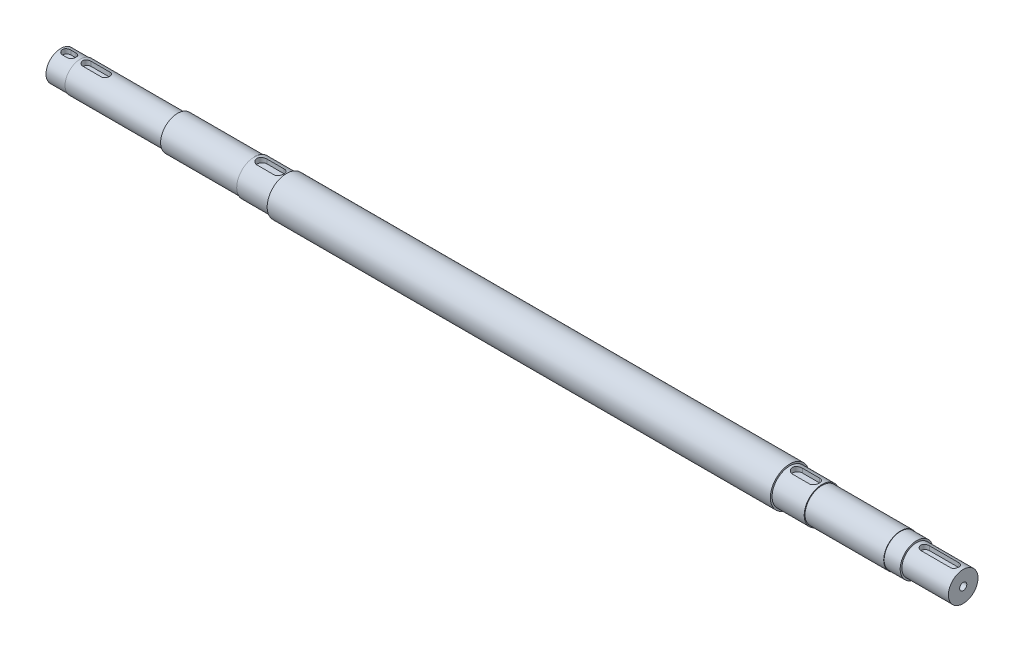
SolidWorks part; units mm, degrees
material "45"
ref_plane "前视基准面" through (0, 0, 0) normal (0, 0, 1) x (1, 0, 0)
ref_plane "上视基准面" through (0, 0, 0) normal (0, 1, 0) x (1, 0, 0)
ref_plane "右视基准面" through (0, 0, 0) normal (1, 0, 0) x (0, 0, -1)
sketch "草图1" plane through (0, 0, 0) normal (1, 0, 0) x (0, 0, -1)
  circle A0 centre (0, 0) radius 23
extrude "凸台-拉伸1" add sketch "草图1" along normal blind 595
sketch "草图2" plane through (0, 0, 0) normal (-1, 0, 0) x (0, 0, 1)
  circle A0 centre (0, 0) radius 21
extrude "凸台-拉伸2" add sketch "草图2" along normal blind 38
sketch "草图3" plane through (-38, 0, 0) normal (-1, 0, 0) x (0, 0, 1)
  circle A0 centre (0, 0) radius 20
extrude "凸台-拉伸3" add sketch "草图3" along normal blind 91
sketch "草图4" plane through (-129, 0, 0) normal (-1, 0, 0) x (0, 0, 1)
  circle A0 centre (0, 0) radius 18
extrude "凸台-拉伸4" add sketch "草图4" along normal blind 115
sketch "草图5" plane through (-244, 0, 0) normal (-1, 0, 0) x (0, 0, 1)
  circle A0 centre (0, 0) radius 17.5
extrude "凸台-拉伸5" add sketch "草图5" along normal blind 23
ref_plane "基准面1" through (0, 21, 0) normal (0, 1, 0) x (1, 0, 0)
sketch "草图6" plane through (0, 21, 0) normal (0, 1, 0) x (1, 0, 0)
  line L0 (-9, 0) -> (-29, 0) construction
  line L1 (-9, -6) -> (-29, -6)
  line L2 (-9, 6) -> (-29, 6)
  line L3 (0, 21) -> (0, -21) construction
  line L4 (604, 0) -> (624, 0) construction
  line L5 (595, -23) -> (595, 23) construction
  line L6 (604, 6) -> (624, 6)
  line L7 (604, -6) -> (624, -6)
  arc A0 (-9, -6) -> (-9, 6) centre (-9, 0) ccw
  arc A1 (-29, 6) -> (-29, -6) centre (-29, 0) ccw
  arc A2 (604, 6) -> (604, -6) centre (604, 0) ccw
  arc A3 (624, -6) -> (624, 6) centre (624, 0) ccw
  point P3 (-19, 0)
  point P14 (614, 0)
  dimension "D1" = 9
  dimension "D2" = 6
  dimension "D4" = 20
  dimension "D5" = 6
  dimension "D3" = 20
  dimension "D6" = 9
sketch "草图7" plane through (595, 0, 0) normal (1, 0, 0) x (0, 0, -1)
  circle A0 centre (0, 0) radius 21
extrude "凸台-拉伸6" add sketch "草图7" along normal blind 38
extrude "切除-拉伸2" cut sketch "草图6" against normal blind 5.88
ref_plane "基准面2" through (0, 18, 0) normal (0, 1, 0) x (1, 0, 0)
sketch "草图9" plane through (0, 18, 0) normal (0, 1, 0) x (1, 0, 0)
  line L0 (-236, 0) -> (-214, 0) construction
  line L1 (-244, 18) -> (-244, -18) construction
  line L2 (-236, 5) -> (-214, 5)
  line L3 (-236, -5) -> (-214, -5)
  arc A0 (-236, 5) -> (-236, -5) centre (-236, 0) ccw
  arc A1 (-214, -5) -> (-214, 5) centre (-214, 0) ccw
  point P5 (-225, 0)
  dimension "D1" = 22
  dimension "D2" = 5
  dimension "D3" = 8
extrude "切除-拉伸3" cut sketch "草图9" against normal blind 6.03
sketch "草图10" plane through (633, 0, 0) normal (1, 0, 0) x (0, 0, -1)
  circle A0 centre (0, 0) radius 20
extrude "凸台-拉伸7" add sketch "草图10" along normal blind 93
sketch "草图11" plane through (726, 0, 0) normal (1, 0, 0) x (0, 0, -1)
  circle A0 centre (0, 0) radius 19.5
extrude "凸台-拉伸8" add sketch "草图11" along normal blind 19
sketch "草图12" plane through (745, 0, 0) normal (1, 0, 0) x (0, 0, -1)
  circle A0 centre (0, 0) radius 17.5
extrude "凸台-拉伸9" add sketch "草图12" along normal blind 55
ref_plane "基准面3" through (0, 17.5, 0) normal (0, 1, 0) x (1, 0, 0)
sketch "草图13" plane through (0, 17.5, 0) normal (0, 1, 0) x (1, 0, 0)
  line L0 (-254, 0) -> (-260, 0) construction
  line L1 (790, 0) -> (755, 0) construction
  line L2 (-254, -5) -> (-260, -5)
  line L3 (-254, 5) -> (-260, 5)
  line L4 (-267, 17.5) -> (-267, -17.5) construction
  line L5 (790, -5) -> (755, -5)
  line L6 (790, 5) -> (755, 5)
  line L7 (745, -17.5) -> (745, 17.5) construction
  arc A0 (-254, -5) -> (-254, 5) centre (-254, 0) ccw
  arc A1 (-260, 5) -> (-260, -5) centre (-260, 0) ccw
  arc A2 (790, -5) -> (790, 5) centre (790, 0) ccw
  arc A3 (755, 5) -> (755, -5) centre (755, 0) ccw
  point P5 (-257, 0)
  point P12 (772.5, 0)
  dimension "D1" = 5
  dimension "D3" = 7
  dimension "D4" = 5
  dimension "D5" = 10
  dimension "D2" = 6
extrude "切除-拉伸4" cut sketch "草图13" against normal blind 5.73
hole_wizard "M10 螺纹孔1" positions "草图15" profile "草图14" tap size "M10" standard "Iso"
sketch "草图15" plane through (-267, 0, 0) normal (-1, 0, 0) x (0, 0, 1)
  point P0 (0, 0)
sketch "草图14" plane through (-267, 0, 0) normal (0, 1, 0) x (0, 0, 1)
  line L0 (0, 0) -> (0, 17.5537)
  line L1 (0, 17.5537) -> (4.25, 15)
  line L2 (4.25, 15) -> (4.25, 0)
  line L5 (4.25, 0) -> (0, 0)
  line L10 (0, 17.5537) -> (-4.25, 15) construction
  line L11 (0, -6.35) -> (0, 107.95) construction
  dimension "螺纹孔钻头直径" = 8.5
  dimension "螺纹孔钻头深度" = 15
  dimension "导头角度" = 118
cosmetic thread "孔螺蚊线1" parameters "D1"=15, "D2"=10
hole_wizard "M10 螺纹孔2" positions "草图17" profile "草图16" tap size "M10" standard "Iso"
sketch "草图17" plane through (800, 0, 0) normal (1, 0, 0) x (0, 0, -1)
  point P0 (0, 0)
sketch "草图16" plane through (800, 0, 0) normal (0, 1, 0) x (0, 0, -1)
  line L0 (0, 0) -> (0, 17.5537)
  line L1 (0, 17.5537) -> (4.25, 15)
  line L2 (4.25, 15) -> (4.25, 0)
  line L5 (4.25, 0) -> (0, 0)
  line L10 (0, 17.5537) -> (-4.25, 15) construction
  line L11 (0, -6.35) -> (0, 107.95) construction
  dimension "螺纹孔钻头直径" = 8.5
  dimension "螺纹孔钻头深度" = 15
  dimension "导头角度" = 118
cosmetic thread "孔螺蚊线2" parameters "D1"=15, "D2"=10
mirror "镜向1" about plane through (0, 0, 0) normal (0, 1, 0) of "切除-拉伸3"
